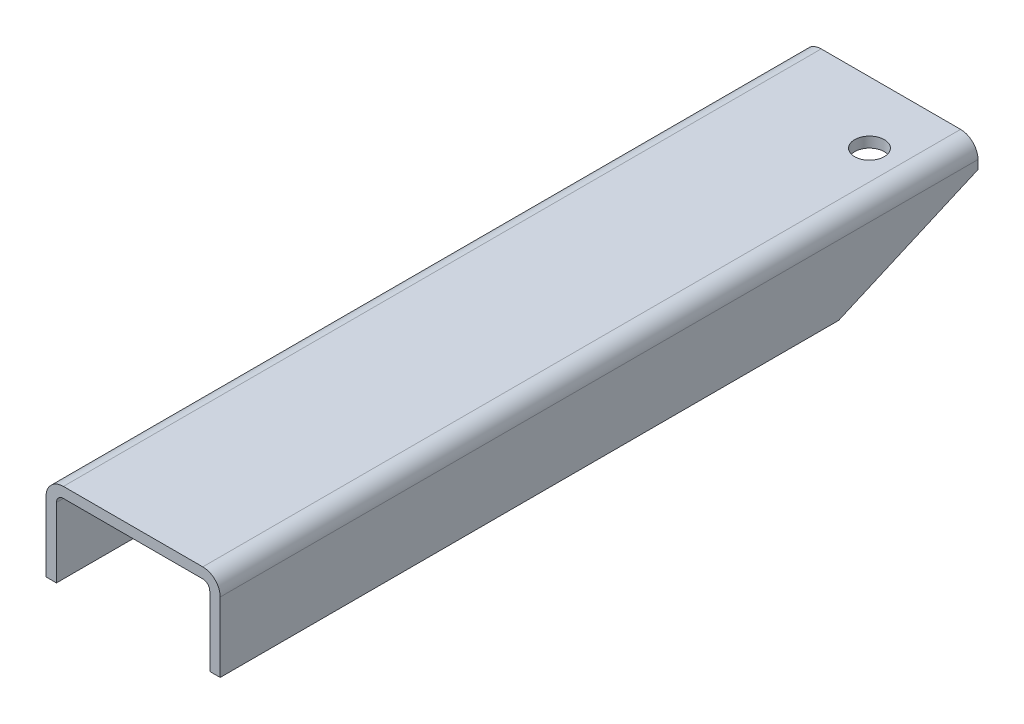
SolidWorks part; units mm, degrees
material "1023 Carbon Steel Plate (SS)"
ref_plane "Front Plane" through (0, 0, 0) normal (0, 0, 1) x (1, 0, 0)
ref_plane "Top Plane" through (0, 0, 0) normal (0, 1, 0) x (1, 0, 0)
ref_plane "Right Plane" through (0, 0, 0) normal (1, 0, 0) x (0, 0, -1)
sketch "Sketch1" plane through (0, 0, 0) normal (0, 0, 1) x (1, 0, 0)
  line L0 (0, 0) -> (0, 40)
  line L1 (10, 50) -> (90, 50)
  line L2 (100, 40) -> (100, 0)
  line L3 (6, 0) -> (6, 40)
  line L4 (10, 44) -> (90, 44)
  line L5 (94, 40) -> (94, 0)
  line L6 (6, 0) -> (0, 0)
  line L7 (100, 0) -> (94, 0)
  arc A0 (90, 50) -> (100, 40) centre (90, 40) cw
  arc A1 (0, 40) -> (10, 50) centre (10, 40) cw
  arc A2 (6, 40) -> (10, 44) centre (10, 40) cw
  arc A3 (90, 44) -> (94, 40) centre (90, 40) cw
  point P7 (100, 50)
  point P10 (0, 50)
  dimension "D4" = 10
  dimension "D1" = 50
  dimension "D2" = 100
  dimension "D3" = 50
  dimension "D5" = 6
extrude "Boss-Extrude1" add sketch "Sketch1" along normal blind 435 contours L7 L5 A3 L4 A2 L3 L6 L0 A1 L1 A0 L2
sketch "Sketch2" plane through (0, 50, 0) normal (0, 1, 0) x (1, 0, 0)
  line L0 (0, -435) -> (0, 0) construction
  line L1 (10, -435) -> (90, -435) construction
  circle A0 centre (73.2, -35.5) radius 8.5
  dimension "D1" = 73.2
  dimension "D2" = 399.5
  dimension "D3" = 17
extrude "Cut-Extrude1" cut sketch "Sketch2" against normal blind 435
sketch "Sketch3" plane through (100, 0, 0) normal (1, 0, 0) x (0, 0, -1)
  line L0 (-80, 0) -> (0, 35)
  line L1 (-435, 0) -> (0, 0) construction
  line L2 (0, 40) -> (0, 0) construction
  line L3 (0, 35) -> (0, 0)
  line L4 (0, 0) -> (-80, 0)
  dimension "D1" = 80
  dimension "D2" = 35
extrude "Cut-Extrude2" cut sketch "Sketch3" against normal blind 435
